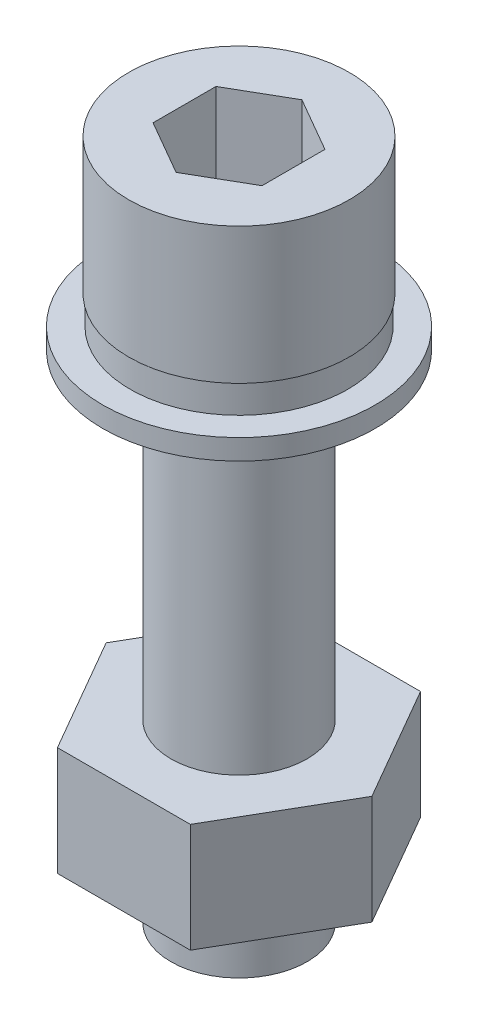
SolidWorks part; units mm, degrees
ref_plane "Front Plane" through (0, 0, 0) normal (0, 0, 1) x (1, 0, 0)
ref_plane "Top Plane" through (0, 0, 0) normal (0, 1, 0) x (1, 0, 0)
ref_plane "Right Plane" through (0, 0, 0) normal (1, 0, 0) x (0, 0, -1)
sketch "Sketch 1" plane through (0, 0, 0) normal (0, 0, 1) x (1, 0, 0)
  line L0 (0, 11.322) -> (0, -25.8305) construction
  line L1 (-9.8983, 0) -> (13.1525, 0) construction
  line L2 (0, 10) -> (-8.1, 10)
  line L3 (-8.1, 10) -> (-8.1, 0)
  line L4 (-8.1, 0) -> (-5, 0)
  line L5 (-5, 0) -> (-5, -40)
  line L6 (-5, -40) -> (0, -40)
  line L7 (0, -40) -> (0, 10)
  dimension "D1" = 10
  dimension "D2" = 40
  dimension "D3" = 10
  dimension "D4" = 16.2
revolve "Revolve 1" add sketch "Sketch 1" angle 360 about L0
sketch "Sketch 2" plane through (0, 10, 0) normal (0, 1, 0) x (1, 0, 0)
  line L1 (0, 4.6188) -> (-4, 2.3094)
  line L2 (-4, 2.3094) -> (-4, -2.3094)
  line L3 (-4, -2.3094) -> (0, -4.6188)
  line L4 (0, -4.6188) -> (4, -2.3094)
  line L5 (4, -2.3094) -> (4, 2.3094)
  line L6 (4, 2.3094) -> (0, 4.6188)
  circle A0 centre (0, 0) radius 4 construction
  dimension "D1" = 8
extrude "Cut-Extrude 1" cut sketch "Sketch 2" against normal blind 6
sketch "Sketch 3" plane through (0, 0, 0) normal (0, -1, 0) x (1, 0, 0)
  circle A0 centre (0, 0) radius 5
  circle A1 centre (0, 0) radius 8
  dimension "D1" = 3
  dimension "D2" = 10
extrude "Boss-Extrude 1" add sketch "Sketch 3" along normal blind 2.1 separate body
sketch "Sketch 4" plane through (0, -2.1, 0) normal (0, -1, 0) x (1, 0, 0)
  circle A0 centre (0, 0) radius 10
  circle A1 centre (0, 0) radius 5
  dimension "D1" = 10
  dimension "D2" = 20
extrude "Boss-Extrude 2" add sketch "Sketch 4" along normal blind 1.5 separate body
ref_plane "Plane 1" through (0, -27.1, 0) normal (0, -1, 0) x (-1, 0, 0)
sketch "Sketch 5" plane through (0, -27.1, 0) normal (0, -1, 0) x (-1, 0, 0)
  line L1 (-9.7572, 0) -> (-4.8786, -8.45)
  line L2 (-4.8786, -8.45) -> (4.8786, -8.45)
  line L3 (4.8786, -8.45) -> (9.7572, 0)
  line L4 (9.7572, 0) -> (4.8786, 8.45)
  line L5 (4.8786, 8.45) -> (-4.8786, 8.45)
  line L6 (-4.8786, 8.45) -> (-9.7572, 0)
  circle A0 centre (0, 0) radius 8.45 construction
  circle A1 centre (0, 0) radius 5
  circle A2 centre (0, 0) radius 5
  dimension "D2" = 16.9
  dimension "D1" = 0
extrude "Boss-Extrude 3" add sketch "Sketch 5" along normal blind 8
